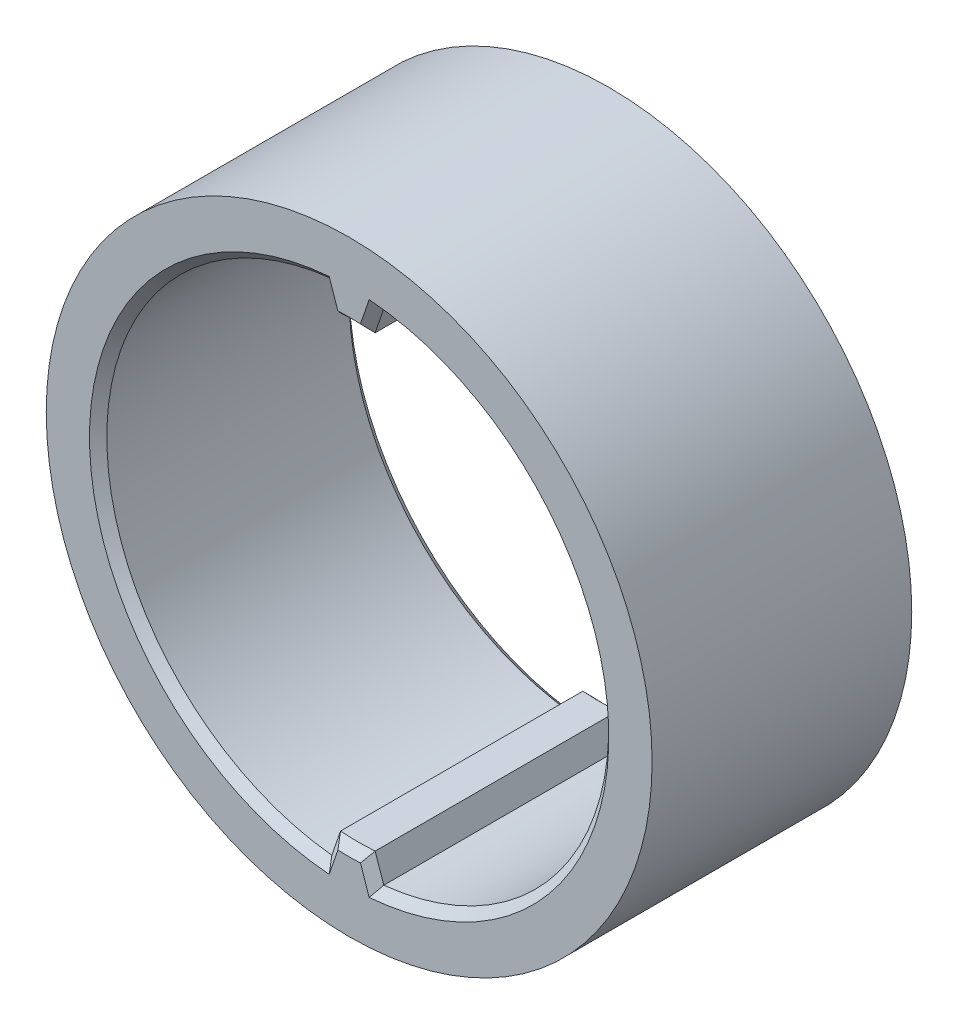
SolidWorks part; units mm, degrees
material "6061 Alloy (GB)"
ref_plane "Front Plane" through (0, 0, 0) normal (0, 0, 1) x (1, 0, 0)
ref_plane "Top Plane" through (0, 0, 0) normal (0, 1, 0) x (1, 0, 0)
ref_plane "Right Plane" through (0, 0, 0) normal (1, 0, 0) x (0, 0, -1)
sketch "Sketch2" plane through (0, 0, 0) normal (0, 0, 1) x (1, 0, 0)
  circle A0 centre (0, 0) radius 14.5
  circle A1 centre (0, 0) radius 17.5
  dimension "D1" = 35
  dimension "D2" = 29
extrude "Boss-Extrude1" add sketch "Sketch2" along normal blind 15
sketch "Sketch4" plane through (0, 0, 0) normal (0, 0, 1) x (1, 0, 0)
  line L0 (0, 0) -> (0, 15.4192) construction
  line L1 (-1.5, 14.4222) -> (-1, 12.9615)
  line L3 (1, 12.9615) -> (1.5, 14.4222)
  line L4 (0, 0) -> (9.2833, 0) construction
  line L5 (1, -12.9615) -> (1.5, -14.4222)
  line L7 (-1.5, -14.4222) -> (-1, -12.9615)
  circle A0 centre (0, 0) radius 14.5 construction
  arc A1 (-1, 12.9615) -> (1, 12.9615) centre (0, 0) cw
  circle A4 centre (0, 0) radius 14.5 construction
  arc A5 (-1.5, -14.4222) -> (1.5, -14.4222) centre (0, 0) ccw
  arc A6 (1.5, 14.4222) -> (-1.5, 14.4222) centre (0, 0) ccw
  arc A7 (-1, -12.9615) -> (1, -12.9615) centre (0, 0) ccw
  dimension "D3" = 26
  dimension "D1" = 2
  dimension "D2" = 3
extrude "Boss-Extrude2" add sketch "Sketch4" along normal up to surface (15 mm away) up to face at (17.5, 0, 15)
chamfer "Chamfer1" distance 0.5 angle 45 16 edges at (1.25, -13.6918, 15) (1.25, -13.6918, 0) (-1.25, -13.6918, 15) (-1.25, -13.6918, 0) (-14.5, 0, 15) (-14.5, 0, 0) (-1.25, 13.6918, 15) (-1.25, 13.6918, 0) (1.25, 13.6918, 15) (1.25, 13.6918, 0) (14.5, 0, 0) (14.5, 0, 15) (0, -13, 15) (0, -13, 0) (0, 13, 15) (0, 13, 0)
